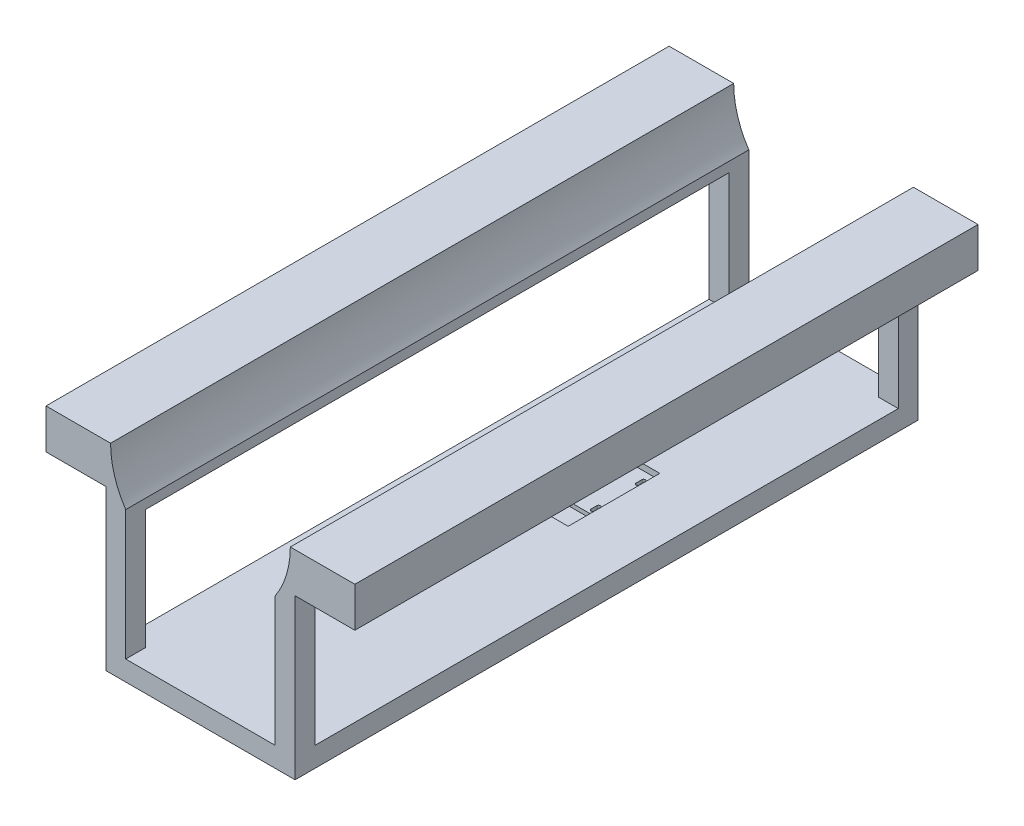
from build123d import *

# Parameters (mm, degrees)
SKETCH_2_W          = 950
SKETCH_2_H          = 3127
EXTRUDE_1_DEPTH     = 1000
SKETCH_4_R          = 451
CUT_EXTRUDE_1_DEPTH = 3708
SKETCH_6_W          = 300
SKETCH_6_H          = 200
EXTRUDE_2_DEPTH     = 3127
SKETCH_9_W          = 750
SKETCH_9_H          = 350
CUT_EXTRUDE_2_DEPTH = 3708
SKETCH_10_W         = 750
SKETCH_10_H         = 3127
CUT_EXTRUDE_3_DEPTH = 3708
CUT_EXTRUDE_4_DEPTH = 50
SKETCH_12_W         = 78.25
SKETCH_12_H         = 300
CUT_EXTRUDE_5_DEPTH = 30
SKETCH_13_W         = 78.25
SKETCH_13_H         = 20
CUT_EXTRUDE_6_DEPTH = 30
SKETCH_14_W         = 160
SKETCH_14_H         = 320
CUT_EXTRUDE_7_DEPTH = 30
SKETCH_15_W         = 2927
SKETCH_15_H         = 600
CUT_EXTRUDE_8_DEPTH = 224
SKETCH_16_W         = 316.5
SKETCH_16_H         = 140
CUT_EXTRUDE_9_DEPTH = 50


with BuildPart() as part:
    # 草图2 → 凸台-拉伸1 (new body)
    with BuildSketch(Plane(origin=(0, 0, 0), x_dir=(1, 0, 0), z_dir=(0, 1, 0))):
        Rectangle(SKETCH_2_W, SKETCH_2_H)
    extrude(amount=-EXTRUDE_1_DEPTH)

    # 草图4 → 切除-拉伸1 (cut)
    with BuildSketch(Plane.XY.offset(1563.5)):
        Circle(SKETCH_4_R)
    extrude(amount=-CUT_EXTRUDE_1_DEPTH, mode=Mode.SUBTRACT)

    # 草图6 → 凸台-拉伸2 (add)
    with BuildSketch(Plane.XY.offset(1563.5)):
        with Locations((-625, -100)):
            Rectangle(SKETCH_6_W, SKETCH_6_H)
        with Locations((625, -100)):
            Rectangle(SKETCH_6_W, SKETCH_6_H)
    extrude(amount=-EXTRUDE_2_DEPTH)

    # 草图9 → 切除-拉伸2 (cut)
    with BuildSketch(Plane.XY.offset(1563.5)):
        with Locations((0, -725)):
            Rectangle(SKETCH_9_W, SKETCH_9_H)
    extrude(amount=-CUT_EXTRUDE_2_DEPTH, mode=Mode.SUBTRACT)

    # 草图10 → 切除-拉伸3 (cut)
    with BuildSketch(Plane(origin=(0, -900, 0), x_dir=(1, 0, 0), z_dir=(0, 1, 0))):
        Rectangle(SKETCH_10_W, SKETCH_10_H)
    extrude(amount=CUT_EXTRUDE_3_DEPTH, mode=Mode.SUBTRACT)

    # 草图11 → 切除-拉伸4 (cut)
    with BuildSketch(Plane(origin=(0, -900, 0), x_dir=(1, 0, 0), z_dir=(0, 1, 0))):
        with BuildLine():
            Line((110.625, 541.5), (110.625, 511.5))
            ThreePointArc((110.625, 511.5), (119.125, 503), (127.625, 511.5))
            Line((127.625, 511.5), (127.625, 541.5))
            ThreePointArc((127.625, 541.5), (119.125, 550), (110.625, 541.5))
        make_face()
        with BuildLine():
            Line((127.625, 315.5), (127.625, 285.5))
            ThreePointArc((127.625, 285.5), (119.125, 277), (110.625, 285.5))
            Line((110.625, 285.5), (110.625, 315.5))
            ThreePointArc((110.625, 315.5), (119.125, 324), (127.625, 315.5))
        make_face()
        with BuildLine():
            Line((-110.625, 285.5), (-110.625, 315.5))
            ThreePointArc((-110.625, 315.5), (-119.125, 324), (-127.625, 315.5))
            Line((-127.625, 315.5), (-127.625, 285.5))
            ThreePointArc((-127.625, 285.5), (-119.125, 277), (-110.625, 285.5))
        make_face()
        with BuildLine():
            Line((-127.625, 511.5), (-127.625, 541.5))
            ThreePointArc((-127.625, 541.5), (-119.125, 550), (-110.625, 541.5))
            Line((-110.625, 541.5), (-110.625, 511.5))
            ThreePointArc((-110.625, 511.5), (-119.125, 503), (-127.625, 511.5))
        make_face()
    extrude(amount=-CUT_EXTRUDE_4_DEPTH, mode=Mode.SUBTRACT)

    # 草图12 → 切除-拉伸5 (cut)
    with BuildSketch(Plane(origin=(0, -900, 0), x_dir=(1, 0, 0), z_dir=(0, 1, 0))):
        with Locations((119.125, 413.5)):
            Rectangle(SKETCH_12_W, SKETCH_12_H)
        with Locations((-119.125, 413.5)):
            Rectangle(SKETCH_12_W, SKETCH_12_H)
    extrude(amount=-CUT_EXTRUDE_5_DEPTH, mode=Mode.SUBTRACT)

    # 草图13 → 切除-拉伸6 (cut)
    with BuildSketch(Plane(origin=(0, -900, 0), x_dir=(1, 0, 0), z_dir=(0, 1, 0))):
        with Locations((119.125, 573.5)):
            Rectangle(SKETCH_13_W, SKETCH_13_H)
        with Locations((-119.125, 573.5)):
            Rectangle(SKETCH_13_W, SKETCH_13_H)
    extrude(amount=-CUT_EXTRUDE_6_DEPTH, mode=Mode.SUBTRACT)

    # 草图14 → 切除-拉伸7 (cut)
    with BuildSketch(Plane(origin=(0, -900, 0), x_dir=(1, 0, 0), z_dir=(0, 1, 0))):
        with Locations((0, 423.5)):
            Rectangle(SKETCH_14_W, SKETCH_14_H)
    extrude(amount=-CUT_EXTRUDE_7_DEPTH, mode=Mode.SUBTRACT)

    # 草图15 → 切除-拉伸8 (cut)
    with BuildSketch(Plane(origin=(475, 0, 0), x_dir=(0, 0, -1), z_dir=(1, 0, 0))):
        with Locations((0, -600)):
            Rectangle(SKETCH_15_W, SKETCH_15_H)
    cut_extrude_8 = extrude(amount=-CUT_EXTRUDE_8_DEPTH, mode=Mode.SUBTRACT)

    # 镜向1: 切除-拉伸8 across plane
    add(cut_extrude_8.mirror(Plane(origin=(0, 0, 0), x_dir=(0, 0, 1), z_dir=(1, 0, 0))), mode=Mode.SUBTRACT)

    # 草图16 → 切除-拉伸9 (cut)
    with BuildSketch(Plane(origin=(0, -900, 0), x_dir=(1, 0, 0), z_dir=(0, 1, 0))):
        with Locations((0, 193.5)):
            Rectangle(SKETCH_16_W, SKETCH_16_H)
    extrude(amount=-CUT_EXTRUDE_9_DEPTH, mode=Mode.SUBTRACT)


solid = part.part
